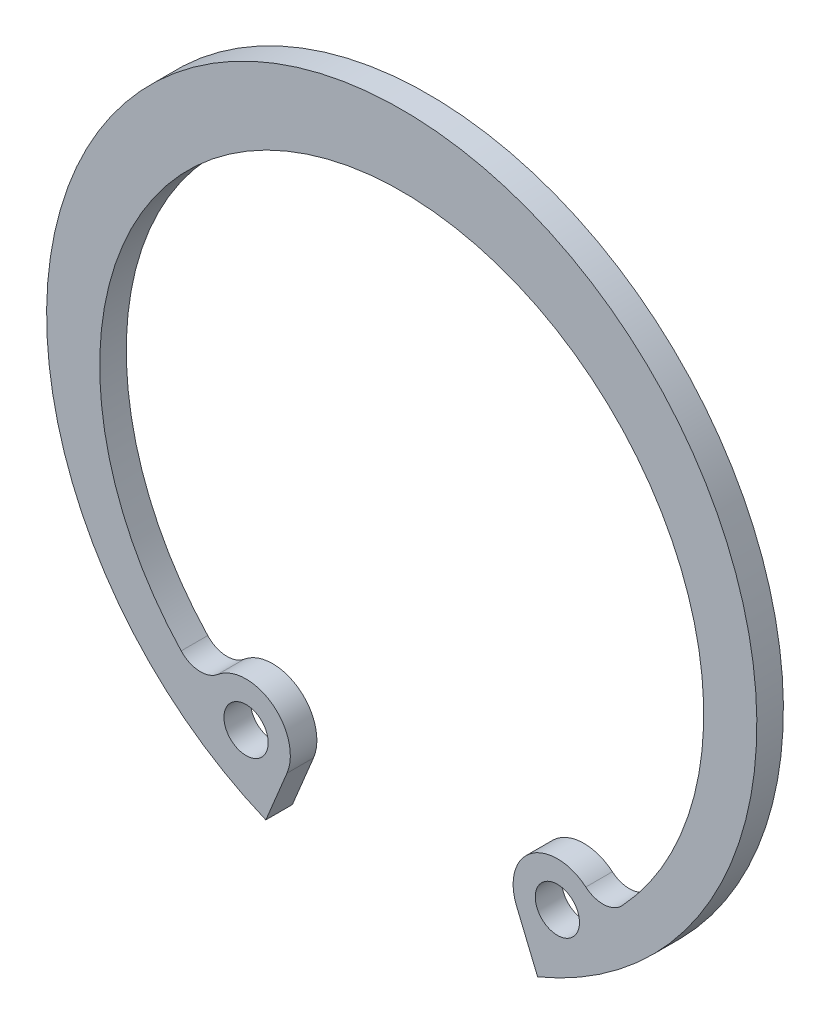
SolidWorks part; units mm, degrees
ref_plane "Front" through (0, 0, 0) normal (0, 0, 1) x (1, 0, 0)
ref_plane "Top" through (0, 0, 0) normal (0, 1, 0) x (1, 0, 0)
ref_plane "Right" through (0, 0, 0) normal (1, 0, 0) x (0, 0, -1)
sketch "Sketch1" plane through (0, 0, 0) normal (0, 0, 1) x (1, 0, 0)
  line L0 (0, 0) -> (-5.1866, -12.5216) construction
  line L1 (0, 7.3554) -> (0, -7.1505) construction
  line L2 (5.1866, -12.5216) -> (6.1421, -14.8283)
  line L4 (-5.1866, -12.5216) -> (-6.1421, -14.8283)
  arc A0 (6.1421, -14.8283) -> (-6.1421, -14.8283) centre (0, 0) ccw
  arc A1 (9.9682, -10.1251) -> (-9.9682, -10.1251) centre (0, -0.8) ccw
  arc A2 (-5.1866, -12.5216) -> (-8.3203, -10.2244) centre (-7.0344, -11.7562) ccw
  arc A3 (-9.9682, -10.1251) -> (-8.3203, -10.2244) centre (-9.0919, -9.3053) ccw
  circle A4 centre (7.0344, -11.7562) radius 1
  arc A5 (9.9682, -10.1251) -> (8.3203, -10.2244) centre (9.0919, -9.3053) cw
  arc A6 (-13.7, 0) -> (13.7, 0) centre (0, 0) ccw construction
  circle A7 centre (-7.0344, -11.7562) radius 1
  arc A8 (5.1866, -12.5216) -> (8.3203, -10.2244) centre (7.0344, -11.7562) cw
  dimension "D" = 32.1
  dimension "d0" = 27.3
  dimension "R1" = 2
  dimension "R2" = 1.2
  dimension "d1" = 2
  dimension "R" = 13.7
  dimension "C" = 0.8
  dimension "Angle" = 45
extrude "Body" add sketch "Sketch1" against normal blind 1.2
